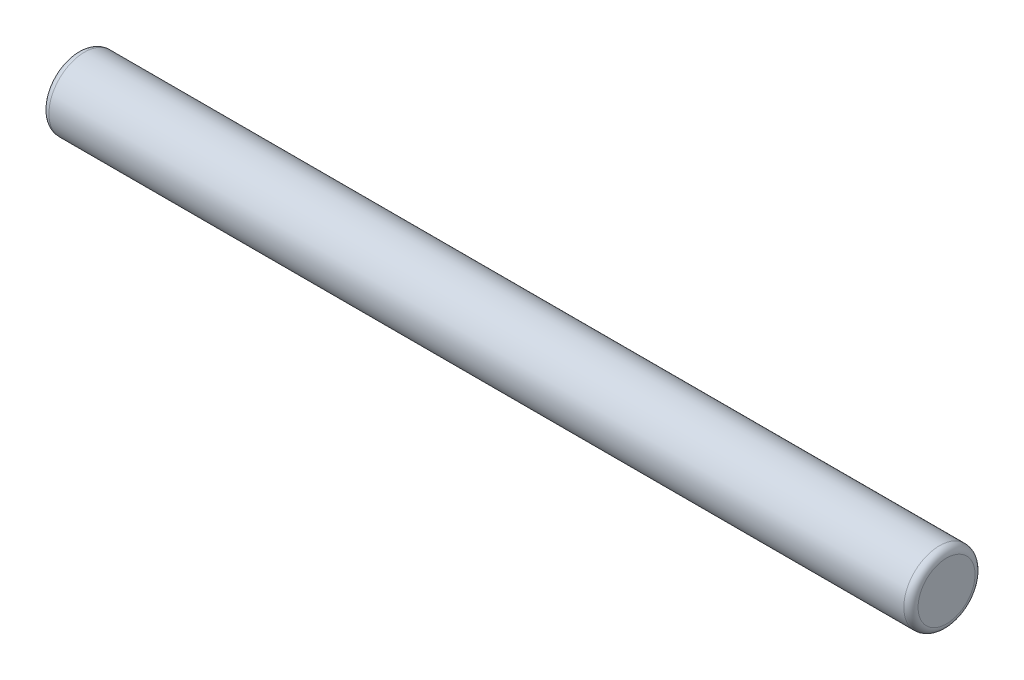
from build123d import *

# Parameters (mm, degrees)
SKETCH_1_R      = 1
EXTRUDE_1_DEPTH = 12.2
FILLET_1_R      = 0.2


with BuildPart() as part:
    # 草图1 → 凸台-拉伸1 (new, symmetric)
    with BuildSketch(Plane(origin=(0, 0, 0), x_dir=(0, 0, -1), z_dir=(1, 0, 0))):
        Circle(SKETCH_1_R)
    extrude(amount=EXTRUDE_1_DEPTH, both=True)

    # 圆角1
    fillet_1_edges = [part.edges().sort_by_distance(p)[0] for p in [
        (-12.2, 0, 1),
        (12.2, 0, 1),
    ]]
    fillet(fillet_1_edges, radius=FILLET_1_R)


solid = part.part
